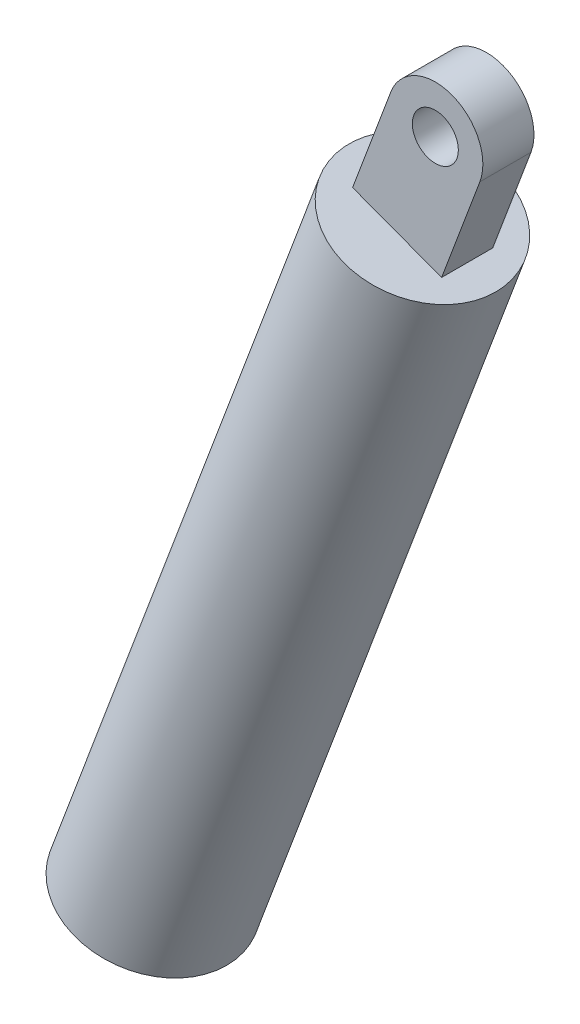
from build123d import *

# Parameters (mm, degrees)
BOSS_EXTRUDE1_DEPTH = 300
BOSS_EXTRUDE2_DEPTH = 20
SKETCH3_R           = 20
CUT_EXTRUDE1_DEPTH  = 260


with BuildPart() as part:
    # Sketch1 → Boss-Extrude1 (new body)
    with BuildSketch(Plane(origin=(135.907089576, 362.468590855, 0), x_dir=(0.9363450005078556, -0.35108124419277087, 0), z_dir=(-0.35108124419277087, -0.9363450005078556, 0))):
        with BuildLine():
            ThreePointArc((546.192823225, 2365.719625064), (515.543416647, 2335.070218486), (546.192823225, 2304.420811908))
            ThreePointArc((546.192823225, 2304.420811908), (576.842229803, 2335.070218486), (546.192823225, 2365.719625064))
        make_face()
    extrude(amount=-BOSS_EXTRUDE1_DEPTH)

    # Sketch2 → Boss-Extrude2 (add)
    with BuildSketch(Plane.XY.offset(2344.984494649)):
        with BuildLine():
            Line((750.199941467, 498.038261237), (735.241534602, 458.143707723))
            Line((735.241534602, 458.143707723), (770.071229746, 445.084362397))
            Line((770.071229746, 445.084362397), (785.029636612, 484.978915911))
            ThreePointArc((785.029636612, 484.978915911), (774.144461703, 508.923436146), (750.199941467, 498.038261237))
        make_face()
        with BuildLine():
            ThreePointArc((760.635963738, 485.825631826), (773.297745788, 484.529763272), (774.593614342, 497.191545322))
            ThreePointArc((774.593614342, 497.191545322), (761.931832291, 498.487413876), (760.635963738, 485.825631826))
        make_face(mode=Mode.SUBTRACT)
    extrude(amount=-BOSS_EXTRUDE2_DEPTH)

    # Sketch3 → Cut-Extrude1 (cut)
    with BuildSketch(Plane(origin=(135.907089576, 362.468590855, 0), x_dir=(0.9363450005078556, -0.351081244192771, 0), z_dir=(-0.351081244192771, -0.9363450005078556, 0))):
        with Locations((546.192823225, 2333.834137652)):
            Circle(SKETCH3_R)
    extrude(amount=-CUT_EXTRUDE1_DEPTH, mode=Mode.SUBTRACT)


solid = part.part
